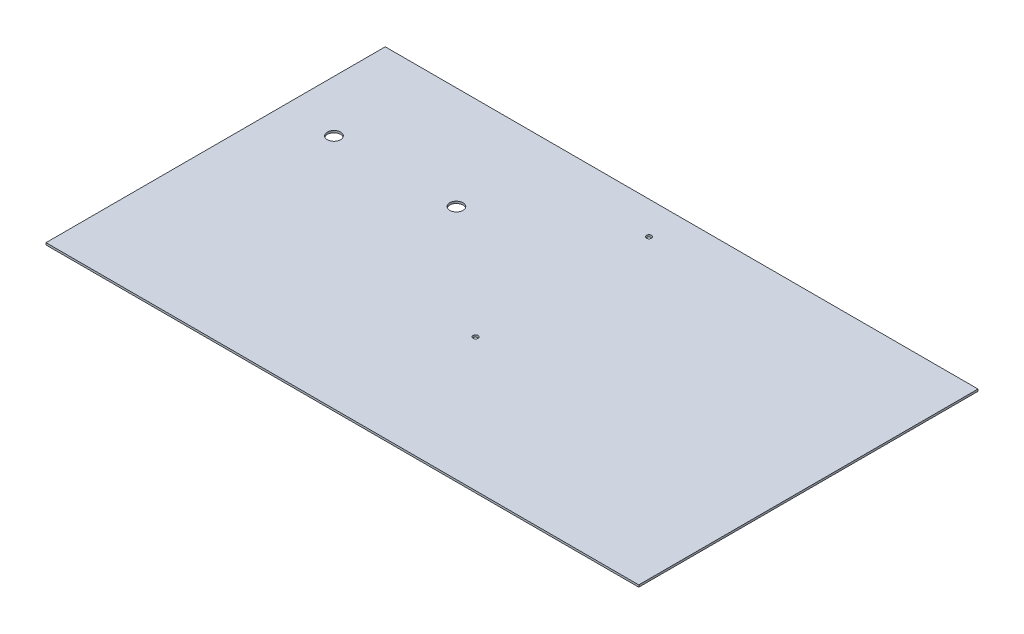
from build123d import *

# Parameters (mm, degrees)
SKETCH_1_W      = 2324
SKETCH_1_H      = 1330
SKETCH_1_R      = 26
SKETCH_1_R_2    = 10
EXTRUDE_1_DEPTH = 4


with BuildPart() as part:
    # 草图1 → 凸台-拉伸1 (new, symmetric)
    with BuildSketch(Plane(origin=(0, 0, 0), x_dir=(1, 0, 0), z_dir=(0, 1, 0))):
        Rectangle(SKETCH_1_W, SKETCH_1_H)
        with Locations(Location((-480, 262, 0), (0, 0, 270))):
            Circle(SKETCH_1_R, mode=Mode.SUBTRACT)
        with Locations(Location((0, 537, 0), (0, 0, 270))):
            Circle(SKETCH_1_R_2, mode=Mode.SUBTRACT)
        with Locations(Location((0, -143, 0), (0, 0, 270))):
            Circle(SKETCH_1_R_2, mode=Mode.SUBTRACT)
        with Locations(Location((-960, 262, 0), (0, 0, 270))):
            Circle(SKETCH_1_R, mode=Mode.SUBTRACT)
    extrude(amount=EXTRUDE_1_DEPTH, both=True)


solid = part.part
